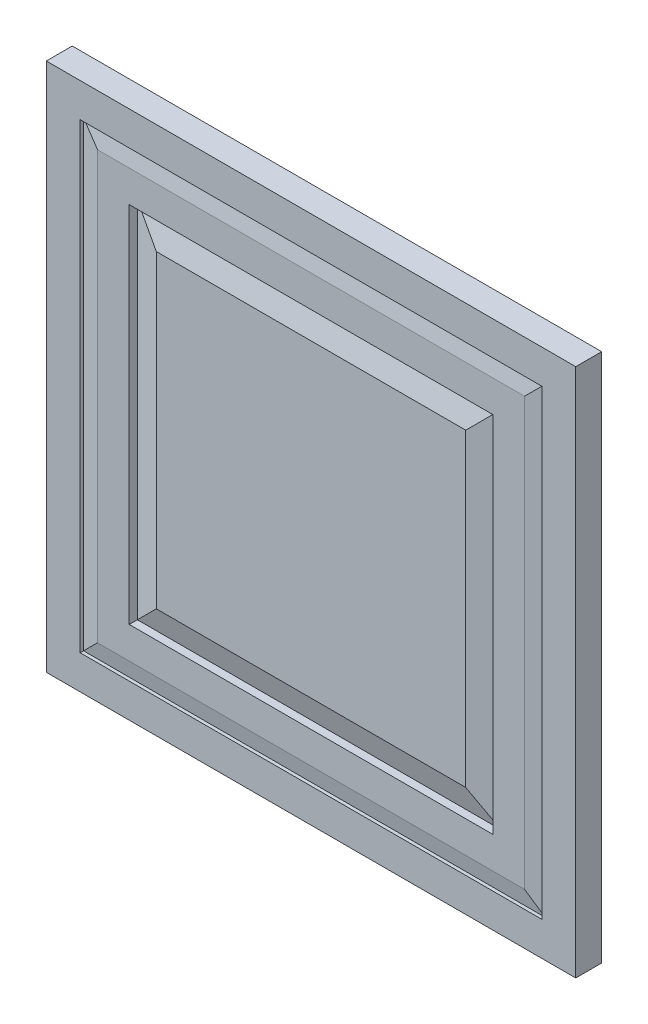
SolidWorks part; units mm, degrees
ref_plane "前视基准面" through (0, 0, 0) normal (0, 0, 1) x (1, 0, 0)
ref_plane "上视基准面" through (0, 0, 0) normal (0, 1, 0) x (1, 0, 0)
ref_plane "右视基准面" through (0, 0, 0) normal (1, 0, 0) x (0, 0, -1)
sketch "草图1" plane through (0, 0, 0) normal (0, 0, 1) x (1, 0, 0)
  line L1 (-102, -102) -> (102, -102)
  line L2 (-102, -102) -> (-102, 102)
  line L3 (-102, 102) -> (102, 102)
  line L4 (102, -102) -> (102, 102)
  line L5 (-102, -102) -> (102, 102) construction
  line L6 (-102, 102) -> (102, -102) construction
  point P0 (0, 0)
  dimension "D1" = 204
  dimension "D2" = 204
extrude "凸台-拉伸1" add sketch "草图1" along normal blind 10
sketch "草图2" plane through (0, 0, 10) normal (0, 0, 1) x (1, 0, 0)
  line L1 (-80, -80) -> (80, -80)
  line L2 (-80, -80) -> (-80, 80)
  line L3 (-80, 80) -> (80, 80)
  line L4 (80, -80) -> (80, 80)
  line L5 (-80, -80) -> (80, 80) construction
  line L6 (-80, 80) -> (80, -80) construction
  point P0 (0, 0)
  dimension "D1" = 160
sketch "草图3" plane through (0, 0, 0) normal (0, 1, 0) x (1, 0, 0)
  line L0 (-88.9483, -10) -> (-88.9483, -8.7052)
  line L1 (102, -10) -> (-102, -10) construction
  line L2 (-88.9483, -8.7052) -> (-82.2706, -10)
  line L3 (-80, -10) -> (80, -10) construction
  line L4 (-88.9483, -10) -> (-82.2706, -10)
sweep "切除-扫描2" cut profiles "草图3" path "草图2"
sketch "草图4" plane through (0, 0, 10) normal (0, 0, 1) x (1, 0, 0)
  line L1 (-70, -70) -> (70, -70)
  line L2 (-70, -70) -> (-70, 70)
  line L3 (-70, 70) -> (70, 70)
  line L4 (70, -70) -> (70, 70)
  line L5 (-70, -70) -> (70, 70) construction
  line L6 (-70, 70) -> (70, -70) construction
  point P0 (0, 0)
  dimension "D1" = 140
sketch "草图5" plane through (0, 0, 0) normal (0, 1, 0) x (1, 0, 0)
  line L0 (-70.0488, -10) -> (-70.0488, -6.8642)
  line L1 (-70, -10) -> (70, -10) construction
  line L2 (-70.0488, -6.8642) -> (-59.6089, -10)
  line L3 (-59.6089, -10) -> (-70.0488, -10)
sweep "切除-扫描3" cut profiles "草图5" path "草图4"
sketch "草图6" plane through (0, 0, 0) normal (0, 0, -1) x (-1, 0, 0)
  line L0 (0, 80.7634) -> (0, 0) construction
  line L1 (0, 0) -> (172.228, 0) construction
  circle A0 centre (-92, 92) radius 2.5
  circle A1 centre (92, 92) radius 2.5
  circle A2 centre (-92, -92) radius 2.5
  circle A3 centre (92, -92) radius 2.5
  dimension "D2" = 184
  dimension "D3" = 5
  dimension "D1" = 184
extrude "切除-拉伸1" cut sketch "草图6" against normal blind 3
sketch "草图7" plane through (0, 0, 0) normal (0, 0, -1) x (-1, 0, 0)
  line L0 (0, 41.5656) -> (0, 0) construction
  line L1 (-86.5, 86.5) -> (86.5, 86.5)
  line L2 (-86.5, 86.5) -> (-86.5, -86.5)
  line L3 (-86.5, -86.5) -> (86.5, -86.5)
  line L4 (86.5, 86.5) -> (86.5, -86.5)
  line L5 (0, 0) -> (60.2041, 0) construction
  dimension "D1" = 173
  dimension "D2" = 173
extrude "凸台-拉伸2" add sketch "草图7" along normal blind 10
